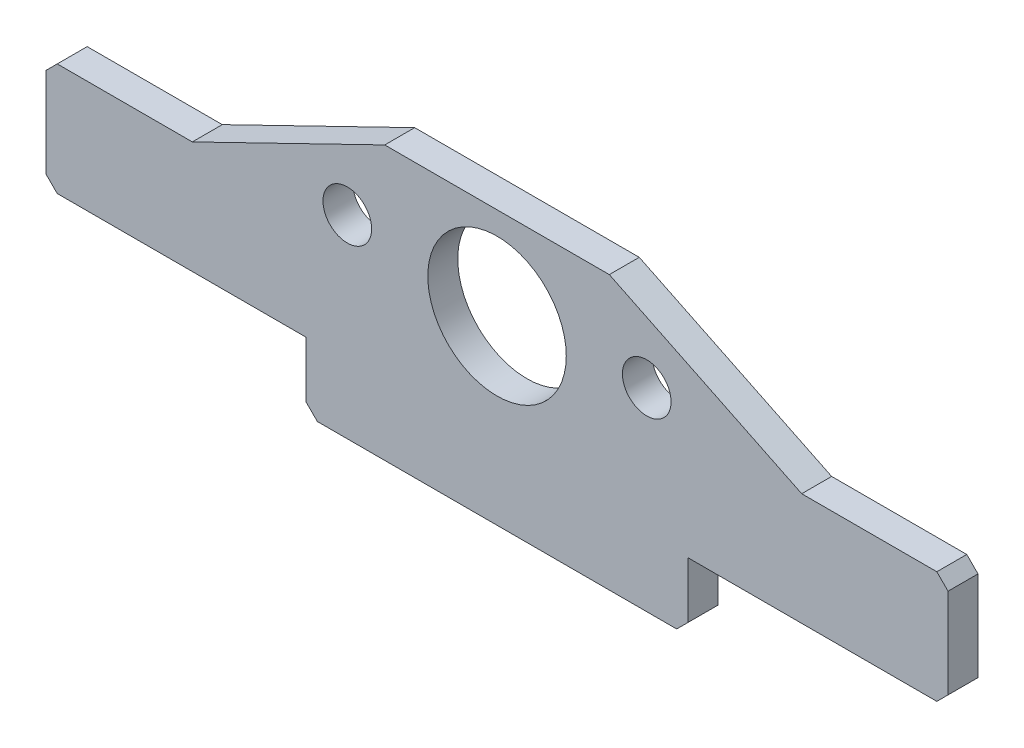
SolidWorks part; units mm, degrees
material "Q235"
ref_plane "Front Plane" through (0, 0, 0) normal (0, 0, 1) x (1, 0, 0)
ref_plane "Top Plane" through (0, 0, 0) normal (0, 1, 0) x (1, 0, 0)
ref_plane "Right Plane" through (0, 0, 0) normal (1, 0, 0) x (0, 0, -1)
sketch "Sketch1" plane through (0, 0, 0) normal (0, 0, 1) x (1, 0, 0)
  line L0 (240, 0) -> (-240, 0)
  line L1 (-255, 15) -> (-255, 90)
  line L2 (-255, 90) -> (-587.5, 90)
  line L3 (-602.5, 105) -> (-602.5, 225)
  line L4 (-587.5, 240) -> (-407, 240)
  line L5 (-407, 240) -> (-150, 365)
  line L6 (-150, 365) -> (150, 365)
  line L7 (0, 365) -> (0, 0) construction
  line L8 (407, 240) -> (150, 365)
  line L9 (587.5, 240) -> (407, 240)
  line L10 (602.5, 105) -> (602.5, 225)
  line L11 (255, 90) -> (587.5, 90)
  line L12 (255, 15) -> (255, 90)
  line L13 (-602.5, 225) -> (-587.5, 240)
  line L14 (-587.5, 90) -> (-602.5, 105)
  line L15 (602.5, 225) -> (587.5, 240)
  line L16 (587.5, 90) -> (602.5, 105)
  line L17 (240, 0) -> (255, 15)
  line L18 (-240, 0) -> (-255, 15)
  circle A0 centre (-200, 259) radius 32.5
  circle A1 centre (200, 259) radius 32.5
  circle A2 centre (0, 242) radius 92.5
  point P1 (-255, 0)
  point P5 (-602.5, 90)
  point P6 (-602.5, 240)
  point P15 (602.5, 240)
  point P16 (602.5, 90)
  point P18 (255, 0)
  dimension "D4" = 106
  dimension "D5" = 65
  dimension "D6" = 400
  dimension "D11" = 123
  dimension "D12" = 185
  dimension "D1" = 510
  dimension "D2" = 1205
  dimension "D3" = 365
  dimension "D7" = 150
  dimension "D8" = 90
  dimension "D9" = 814
  dimension "D10" = 300
extrude "Boss-Extrude1" add sketch "Sketch1" along normal blind 40
